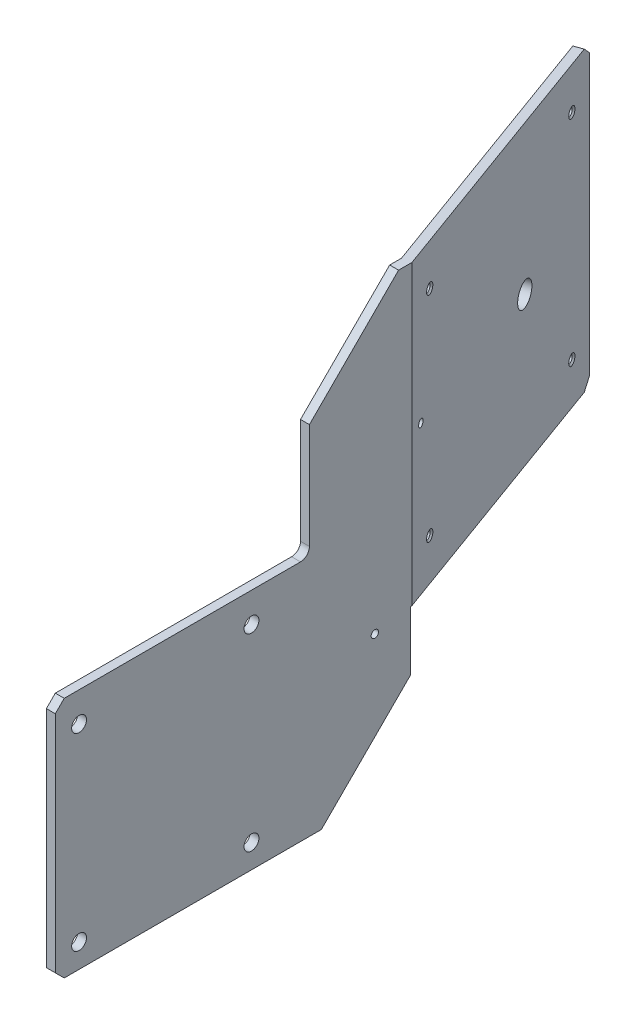
SolidWorks part; units mm, degrees
ref_plane "Front Plane" through (0, 0, 0) normal (0, 0, 1) x (1, 0, 0)
ref_plane "Top Plane" through (0, 0, 0) normal (0, 1, 0) x (1, 0, 0)
ref_plane "Right Plane" through (0, 0, 0) normal (1, 0, 0) x (0, 0, -1)
sketch "Sketch1" plane through (0, 0, 0) normal (0, 1, 0) x (1, 0, 0)
  line L0 (0, 120) -> (-34.202, 213.9693)
  line L1 (0, 0) -> (-3, 0)
  line L2 (0, 0) -> (0, 120)
  line L4 (-3, 0) -> (-3, 119.471)
  line L5 (-34.202, 213.9693) -> (-37.0211, 212.9432)
  line L6 (-37.0211, 212.9432) -> (-3, 119.471)
  dimension "D1" = 3
  dimension "D2" = 3
  dimension "D3" = 20
  dimension "D4" = 120
  dimension "D5" = 100
extrude "Boss-Extrude1" add sketch "Sketch1" along normal blind 100
sketch "Sketch3" plane through (35.7482, 0, -13.0113) normal (-0.9397, 0, 0.342) x (0.342, 0, 0.9397)
  line L0 (-193.9693, 50) -> (49806.0307, 50) construction
  line L1 (-212.7631, 100) -> (-212.7631, 0) construction
  circle A0 centre (-202.7631, 86) radius 1
  circle A1 centre (-202.7631, 14) radius 1
  point P4 (-212.7631, 50)
  dimension "D2" = 2
  dimension "D1" = 72
  dimension "D3" = 10
extrude "Cut-Extrude2" cut sketch "Sketch3" against normal blind 10
pattern_linear "LPattern1" count 2 spacing 80 along (0.342, 0, 0.9397) of "Cut-Extrude2"
hole_wizard "M3 Tapped Hole1" positions "3DSketch1" profile "Sketch4" tap size "M3" standard "Gb"
sketch3d "3DSketch1"
  line L0 (-30.7818, 86, -204.5723) -> (-33.6009, 86, -203.5463) construction
  line L1 (-30.7818, 14, -204.5723) -> (-33.6009, 14, -203.5463) construction
  line L2 (-3.4202, 14, -129.3969) -> (-6.2393, 14, -128.3709) construction
  line L3 (-3.4202, 86, -129.3969) -> (-6.2393, 86, -128.3709) construction
  point P0 (-30.7818, 86, -204.5723)
  point P4 (-30.7818, 14, -204.5723)
  point P8 (-3.4202, 14, -129.3969)
  point P12 (-3.4202, 86, -129.3969)
sketch "Sketch4" plane through (-30.7818, 86, -204.5723) normal (0, 1, 0) x (-0.342, 0, -0.9397)
  line L0 (0, 0) -> (0, 8.2511)
  line L1 (0, 8.2511) -> (1.25, 7.5)
  line L2 (1.25, 7.5) -> (1.25, 0)
  line L5 (1.25, 0) -> (0, 0)
  line L10 (0, 8.2511) -> (-1.25, 7.5) construction
  line L11 (0, -6.35) -> (0, 107.95) construction
  dimension "螺纹孔钻头直径" = 2.5
  dimension "螺纹孔钻头深度" = 7.5
  dimension "导头角度" = 118
cosmetic thread "Hole Thread 1" parameters "D1"=3, "D2"=3
cosmetic thread "Hole Thread 2" parameters "D1"=3, "D2"=3
cosmetic thread "Hole Thread 3" parameters "D1"=3, "D2"=3
cosmetic thread "Hole Thread 4" parameters "D1"=3, "D2"=3
chamfer "Chamfer2" distance 0.5 angle 45 4 edges at (-3.8477, 86, -130.5715) (-3.8477, 14, -130.5715) (-31.2093, 14, -205.747) (-31.2093, 86, -205.747)
sketch "Sketch6" plane through (-3, 0, 0) normal (-1, 0, 0) x (0, 0, 1)
  line L1 (0, 100) -> (-85.5, 100)
  line L2 (0, 100) -> (0, 31.5)
  line L3 (0, 31.5) -> (-85.5, 31.5)
  line L4 (-85.5, 100) -> (-85.5, 31.5)
  dimension "D1" = 68.5
  dimension "D2" = 85.5
extrude "Cut-Extrude4" cut sketch "Sketch6" against normal blind 10
chamfer "Chamfer3" distance 30 angle 45 1 edges at (-1.5, 100, -85.5)
fillet "Fillet1" radius 3 1 edges at (-1.5, 31.5, -85.5)
sketch "Sketch7" plane through (35.7482, 0, -13.0113) normal (-0.9397, 0, 0.342) x (0.342, 0, 0.9397)
  line L0 (-176.2631, 50) -> (-50176.2631, 50) construction
  line L1 (-212.7631, 100) -> (-212.7631, 0) construction
  circle A0 centre (-176.2631, 50) radius 4
  point P8 (-212.7631, 50)
  dimension "D1" = 8
  dimension "D2" = 36.5
extrude "Cut-Extrude5" cut sketch "Sketch7" against normal blind 10
sketch "Sketch9" plane through (-3, 0, 0) normal (-1, 0, 0) x (0, 0, 1)
  line L1 (0, 0) -> (-119.5, 0)
  line L2 (0, 0) -> (0, -50)
  line L3 (0, -50) -> (-119.5, -50)
  line L4 (-119.5, 0) -> (-119.5, -50)
  dimension "D1" = 50
  dimension "D2" = 119.5
extrude "Boss-Extrude2" add sketch "Sketch9" against normal up to surface (3 mm away) up to face at (0, 45.8598, -76.2027)
sketch "Sketch5" plane through (-3, 0, 0) normal (-1, 0, 0) x (0, 0, 1)
  line L1 (-119.5, -50) -> (0, -50) construction
  line L2 (-8, 21.5) -> (-50008, 21.5) construction
  line L3 (0, 31.5) -> (0, -50) construction
  circle A0 centre (-8, 21.5) radius 2.5
  circle A1 centre (-8, -42) radius 2.5
  circle A2 centre (-66, 21.5) radius 2.5
  circle A3 centre (-66, -42) radius 2.5
  dimension "D1" = 58
  dimension "D2" = 8
  dimension "D3" = 5
  dimension "D4" = 63.5
  dimension "D5" = 8
extrude "Cut-Extrude3" cut sketch "Sketch5" against normal blind 10
chamfer "Chamfer4" distance 3 angle 45 4 edges at (-1.5, 31.5, 0) (-35.6116, 100, -213.4562) (-35.6116, 0, -213.4562) (-1.5, -50, 0)
chamfer "Chamfer5" distance 30 angle 45 1 edges at (-1.5, -50, -119.5)
hole_wizard "M3 Tapped Hole2" positions "Sketch11" profile "Sketch10" tap size "M3" standard "Gb"
sketch "Sketch11" plane through (35.7482, 0, -13.0113) normal (-0.9397, 0, 0.342) x (0.342, 0, 0.9397)
  line L0 (-209.7631, 100) -> (-113.2921, 100) construction
  line L1 (-212.7631, 97) -> (-212.7631, 3) construction
  point P0 (-117.7631, 50)
  dimension "D1" = 50
  dimension "D2" = 95
sketch "Sketch10" plane through (-4.5292, 50, -123.6724) normal (0, 1, 0) x (0.342, 0, 0.9397)
  line L0 (0, 0) -> (0, 8.2511)
  line L1 (0, 8.2511) -> (1.25, 7.5)
  line L2 (1.25, 7.5) -> (1.25, 0)
  line L5 (1.25, 0) -> (0, 0)
  line L10 (0, 8.2511) -> (-1.25, 7.5) construction
  line L11 (0, -6.35) -> (0, 107.95) construction
  dimension "螺纹孔钻头直径" = 2.5
  dimension "螺纹孔钻头深度" = 7.5
  dimension "导头角度" = 118
cosmetic thread "Hole Thread 5" parameters "D1"=3, "D2"=3
hole_wizard "M3 Tapped Hole3" positions "Sketch13" profile "Sketch12" tap size "M3" standard "Gb"
sketch "Sketch13" plane through (-3, 0, 0) normal (-1, 0, 0) x (0, 0, 1)
  line L0 (-89.5, -50) -> (-3, -50) construction
  line L1 (-119.5, 0) -> (-119.5, -20) construction
  point P0 (-107.5, -2)
  dimension "D1" = 48
  dimension "D2" = 12
sketch "Sketch12" plane through (-3, -2, -107.5) normal (0, 1, 0) x (0, 0, 1)
  line L0 (0, 0) -> (0, 8.2511)
  line L1 (0, 8.2511) -> (1.25, 7.5)
  line L2 (1.25, 7.5) -> (1.25, 0)
  line L5 (1.25, 0) -> (0, 0)
  line L10 (0, 8.2511) -> (-1.25, 7.5) construction
  line L11 (0, -6.35) -> (0, 107.95) construction
  dimension "螺纹孔钻头直径" = 2.5
  dimension "螺纹孔钻头深度" = 7.5
  dimension "导头角度" = 118
cosmetic thread "Hole Thread 6" parameters "D1"=3, "D2"=3
